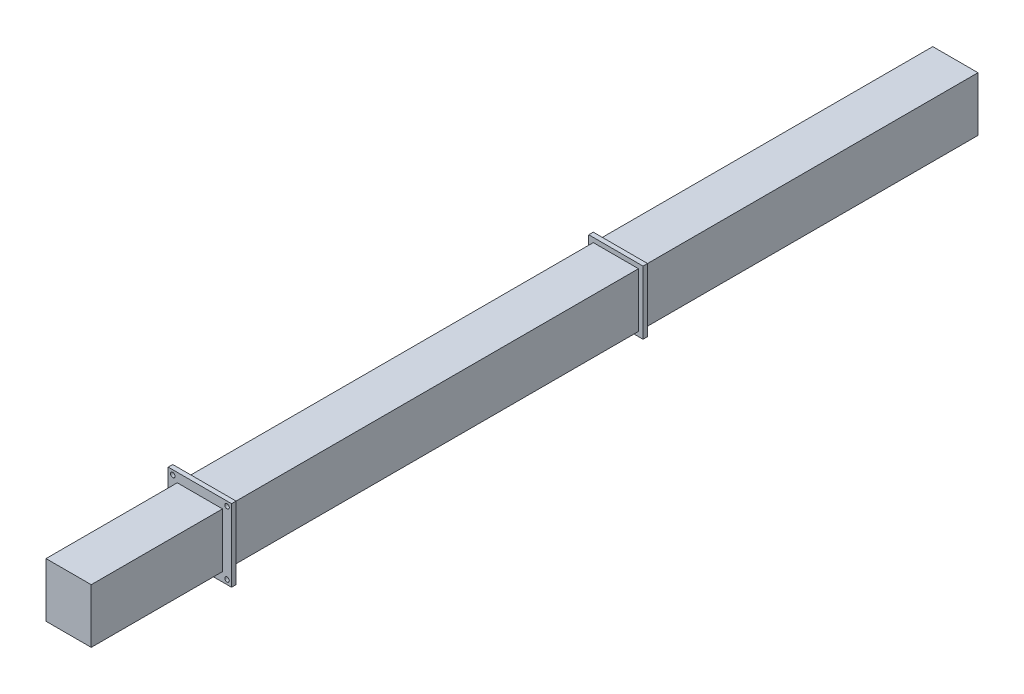
from build123d import *

# Parameters (mm, degrees)
BOSS_EXTRUDE1_DEPTH      = 700
BOSS_EXTRUDE1_DEPTH_BACK = 1259
SKETCH1_W                = 120
SKETCH1_H                = 120
SKETCH2_W                = 20.088480041
SKETCH2_H                = 120
CUT_EXTRUDE1_DEPTH       = 2985
BOSS_EXTRUDE2_START      = -750
SKETCH3_W                = 119.911519959
SKETCH3_H                = 140
BOSS_EXTRUDE2_DEPTH      = 10
BOSS_EXTRUDE3_START      = -300
SKETCH4_W                = 139.911519959
SKETCH4_H                = 160
BOSS_EXTRUDE3_DEPTH      = 10
SKETCH5_R                = 5
CUT_EXTRUDE2_DEPTH       = 10


with BuildPart() as part:
    # Sketch1 → Boss-Extrude1 (new, two sides: drawn at the far end of the back side and taken through both)
    with BuildSketch(Plane.XY.offset(-BOSS_EXTRUDE1_DEPTH_BACK)):
        with Locations((0, 160)):
            Rectangle(SKETCH1_W, SKETCH1_H)
    extrude(amount=BOSS_EXTRUDE1_DEPTH + BOSS_EXTRUDE1_DEPTH_BACK)

    # Sketch2 → Cut-Extrude1 (cut)
    with BuildSketch(Plane.XY.offset(700)):
        with Locations((-49.95575998, 160)):
            Rectangle(SKETCH2_W, SKETCH2_H)
    extrude(amount=-CUT_EXTRUDE1_DEPTH, mode=Mode.SUBTRACT)

    # Sketch3 → Boss-Extrude2 (add)
    with BuildSketch(Plane(origin=(0, 0, -1259), x_dir=(-1, 0, 0), z_dir=(0, 0, -1)).offset(BOSS_EXTRUDE2_START)):
        with Locations((-10.04424002, 160)):
            Rectangle(SKETCH3_W, SKETCH3_H)
    extrude(amount=BOSS_EXTRUDE2_DEPTH)

    # Sketch4 → Boss-Extrude3 (add)
    with BuildSketch(Plane.XY.offset(700).offset(BOSS_EXTRUDE3_START)):
        with Locations((10.04424002, 160)):
            Rectangle(SKETCH4_W, SKETCH4_H)
    extrude(amount=BOSS_EXTRUDE3_DEPTH)

    # Sketch5 → Cut-Extrude2 (cut)
    with BuildSketch(Plane.XY.offset(410)):
        with Locations((70, 230)):
            Circle(SKETCH5_R)
        with Locations((70, 90)):
            Circle(SKETCH5_R)
        with Locations((-49.911519959, 90)):
            Circle(SKETCH5_R)
        with Locations((-49.911519959, 230)):
            Circle(SKETCH5_R)
    extrude(amount=-CUT_EXTRUDE2_DEPTH, mode=Mode.SUBTRACT)


solid = part.part
